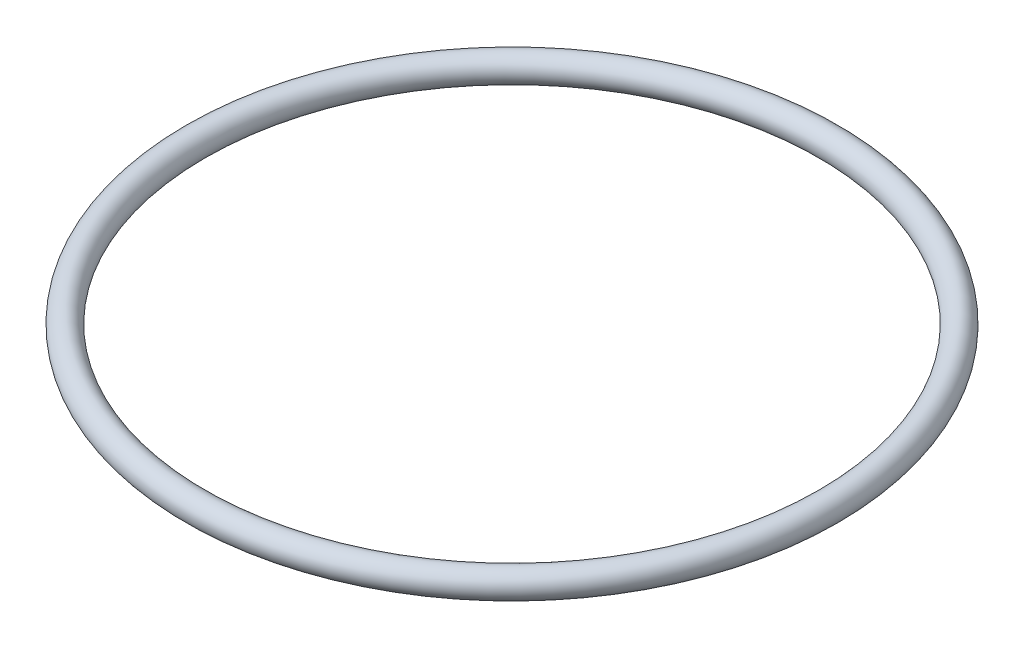
SolidWorks part; units mm, degrees
material "1.4000 (X6Cr13)"
ref_plane "Front Plane" through (0, 0, 0) normal (0, 0, 1) x (1, 0, 0)
ref_plane "Top Plane" through (0, 0, 0) normal (0, 1, 0) x (1, 0, 0)
ref_plane "Right Plane" through (0, 0, 0) normal (1, 0, 0) x (0, 0, -1)
sketch "Sketch1" plane through (0, 0, 0) normal (0, 0, 1) x (1, 0, 0)
  line L0 (-87.5312, -104.0167) -> (-86.0312, -104.0167) construction
  line L1 (-87.5312, -105.6167) -> (-87.5312, -102.4167) construction
  line L2 (-121.5312, -142.3167) -> (-121.5312, 27.192) construction
  line L3 (-142.9055, -142.3167) -> (-100.1568, -142.3167) construction
  line L4 (-121.5312, -131.3167) -> (-121.5312, -142.3167) construction
  circle A0 centre (-86.0312, -104.0167) radius 1.5
  dimension "D1" = 3
  dimension "D2" = 1.5
revolve "Revolve1" add sketch "Sketch1" angle 360 about L2
